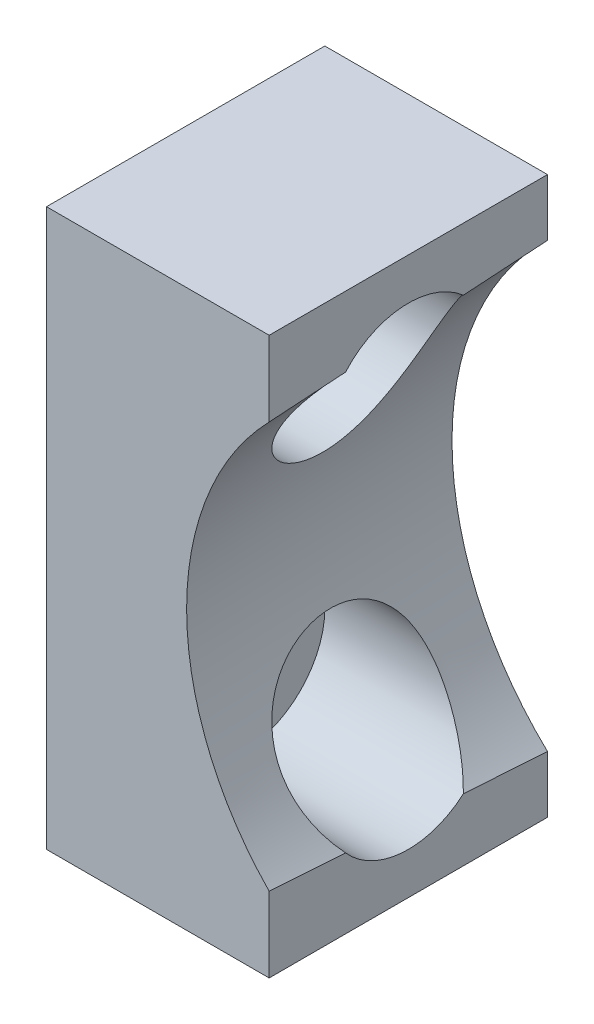
from build123d import *

# Parameters (mm, degrees)
SKETCH_1_W                   = 8
SKETCH_1_H                   = 20
EXTRUDE_1_DEPTH              = 10
HOLE_WIZARD_M3_1_D           = 3.4
HOLE_WIZARD_M3_1_CBORE_D     = 6
HOLE_WIZARD_M3_1_CBORE_DEPTH = 6


with BuildPart() as part:
    # 草图1 → 凸台-拉伸1 (new body)
    with BuildSketch(Plane.XY):
        Rectangle(SKETCH_1_W, SKETCH_1_H)
    extrude(amount=EXTRUDE_1_DEPTH)

    # M3 六角圆柱头螺钉的柱形沉头孔1 (through all)
    with Locations(Plane(origin=(4, 0, 0), x_dir=(0, 0, -1), z_dir=(1, 0, 0))):
        with Locations((-5, 5.5), (-5, -5.5)):
            CounterBoreHole(HOLE_WIZARD_M3_1_D / 2, HOLE_WIZARD_M3_1_CBORE_D / 2, HOLE_WIZARD_M3_1_CBORE_DEPTH)

    # 草图4 → 切除-旋转1 (revolve, cut)
    with BuildSketch(Plane(origin=(0, 0, 0), x_dir=(1, 0, 0), z_dir=(0, 1, 0))):
        Polygon((11.5, 1.5), (0.5, 1.5), (1.200682375, -13.581690109), (11.5, -13.581690109), align=None)
    revolve(axis=Axis((11.5, 0, 13.581690109), (0, 0, -1)), mode=Mode.SUBTRACT)


solid = part.part
